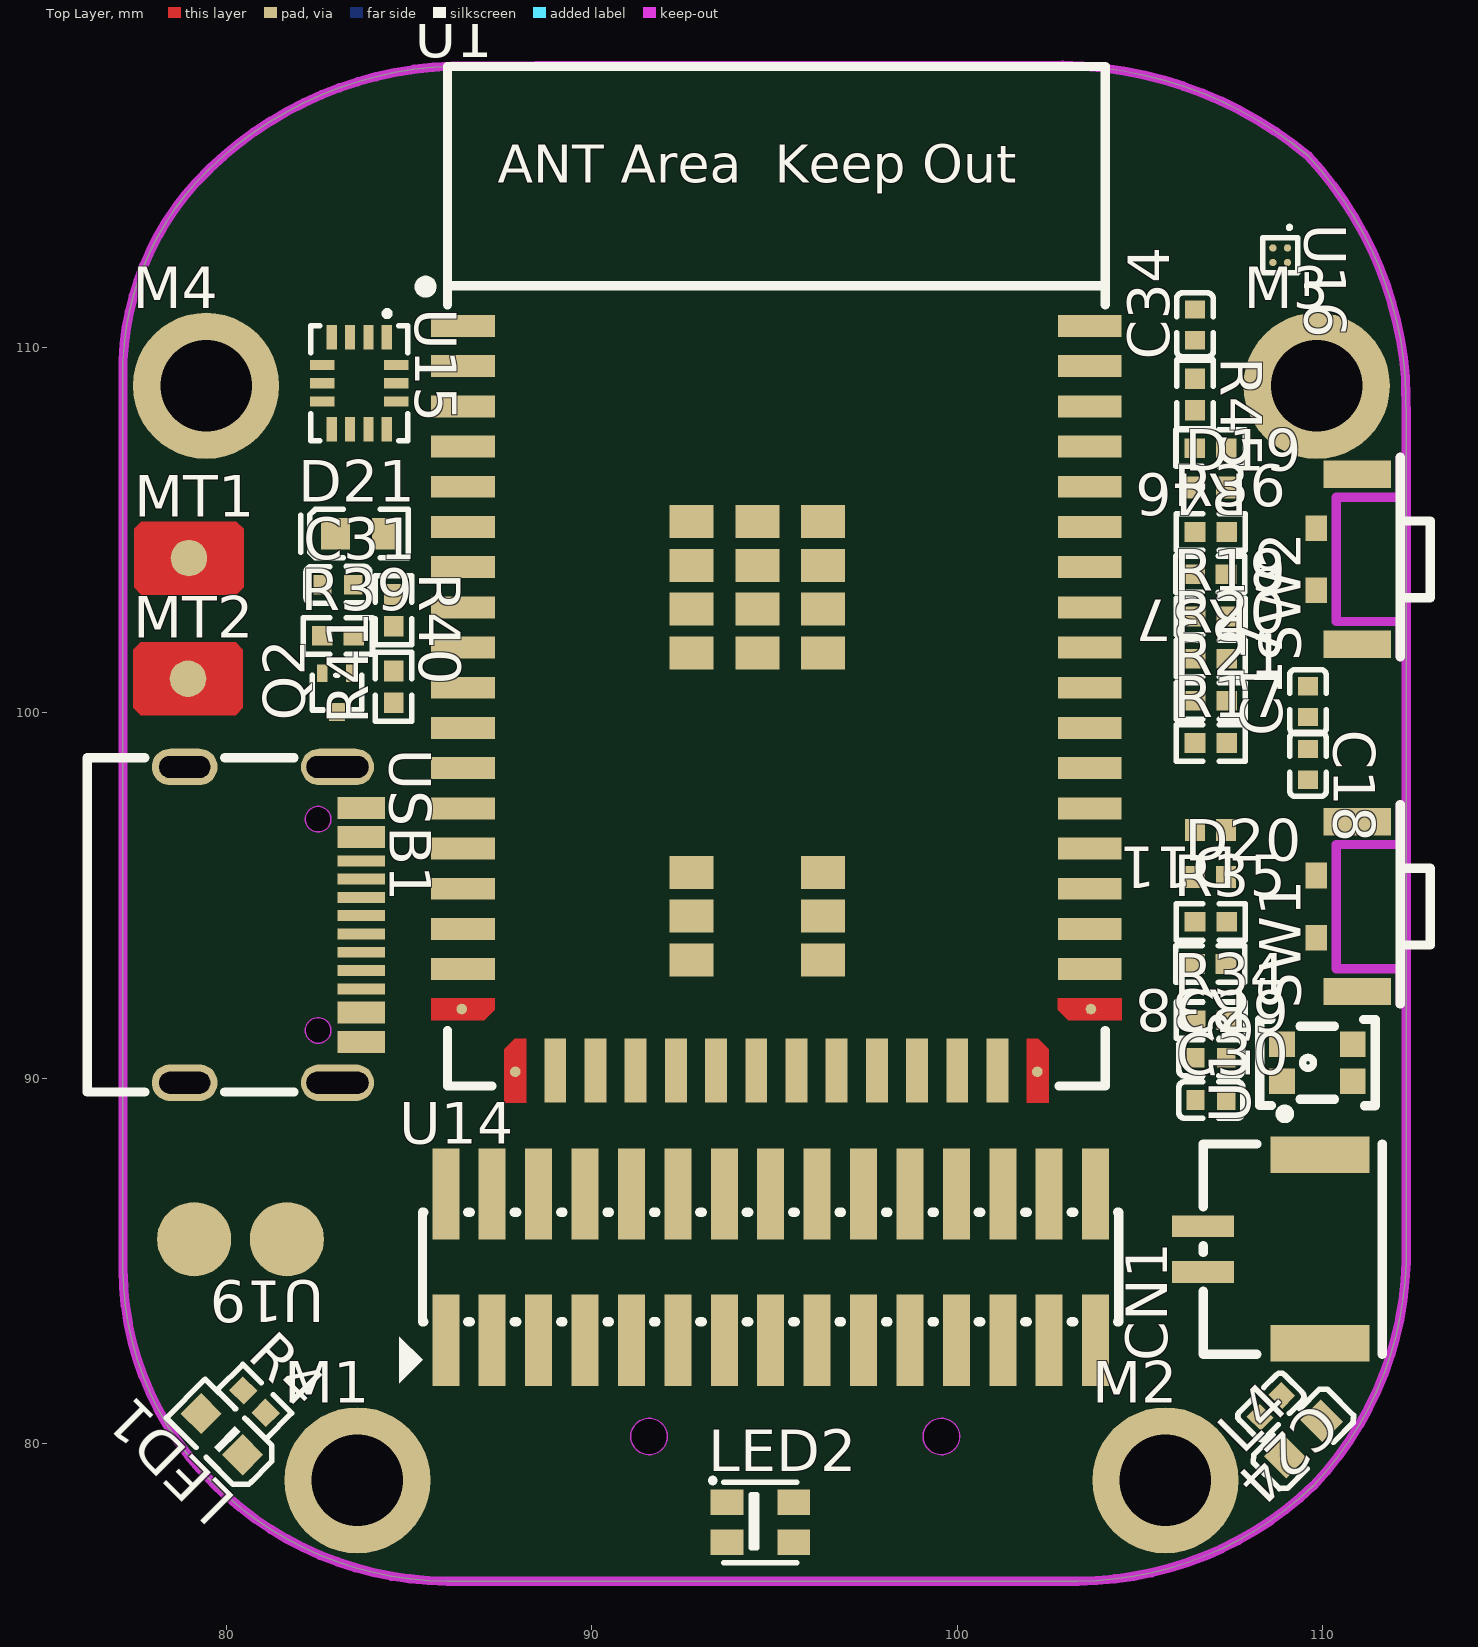
[diagram p0: Top Layer view]
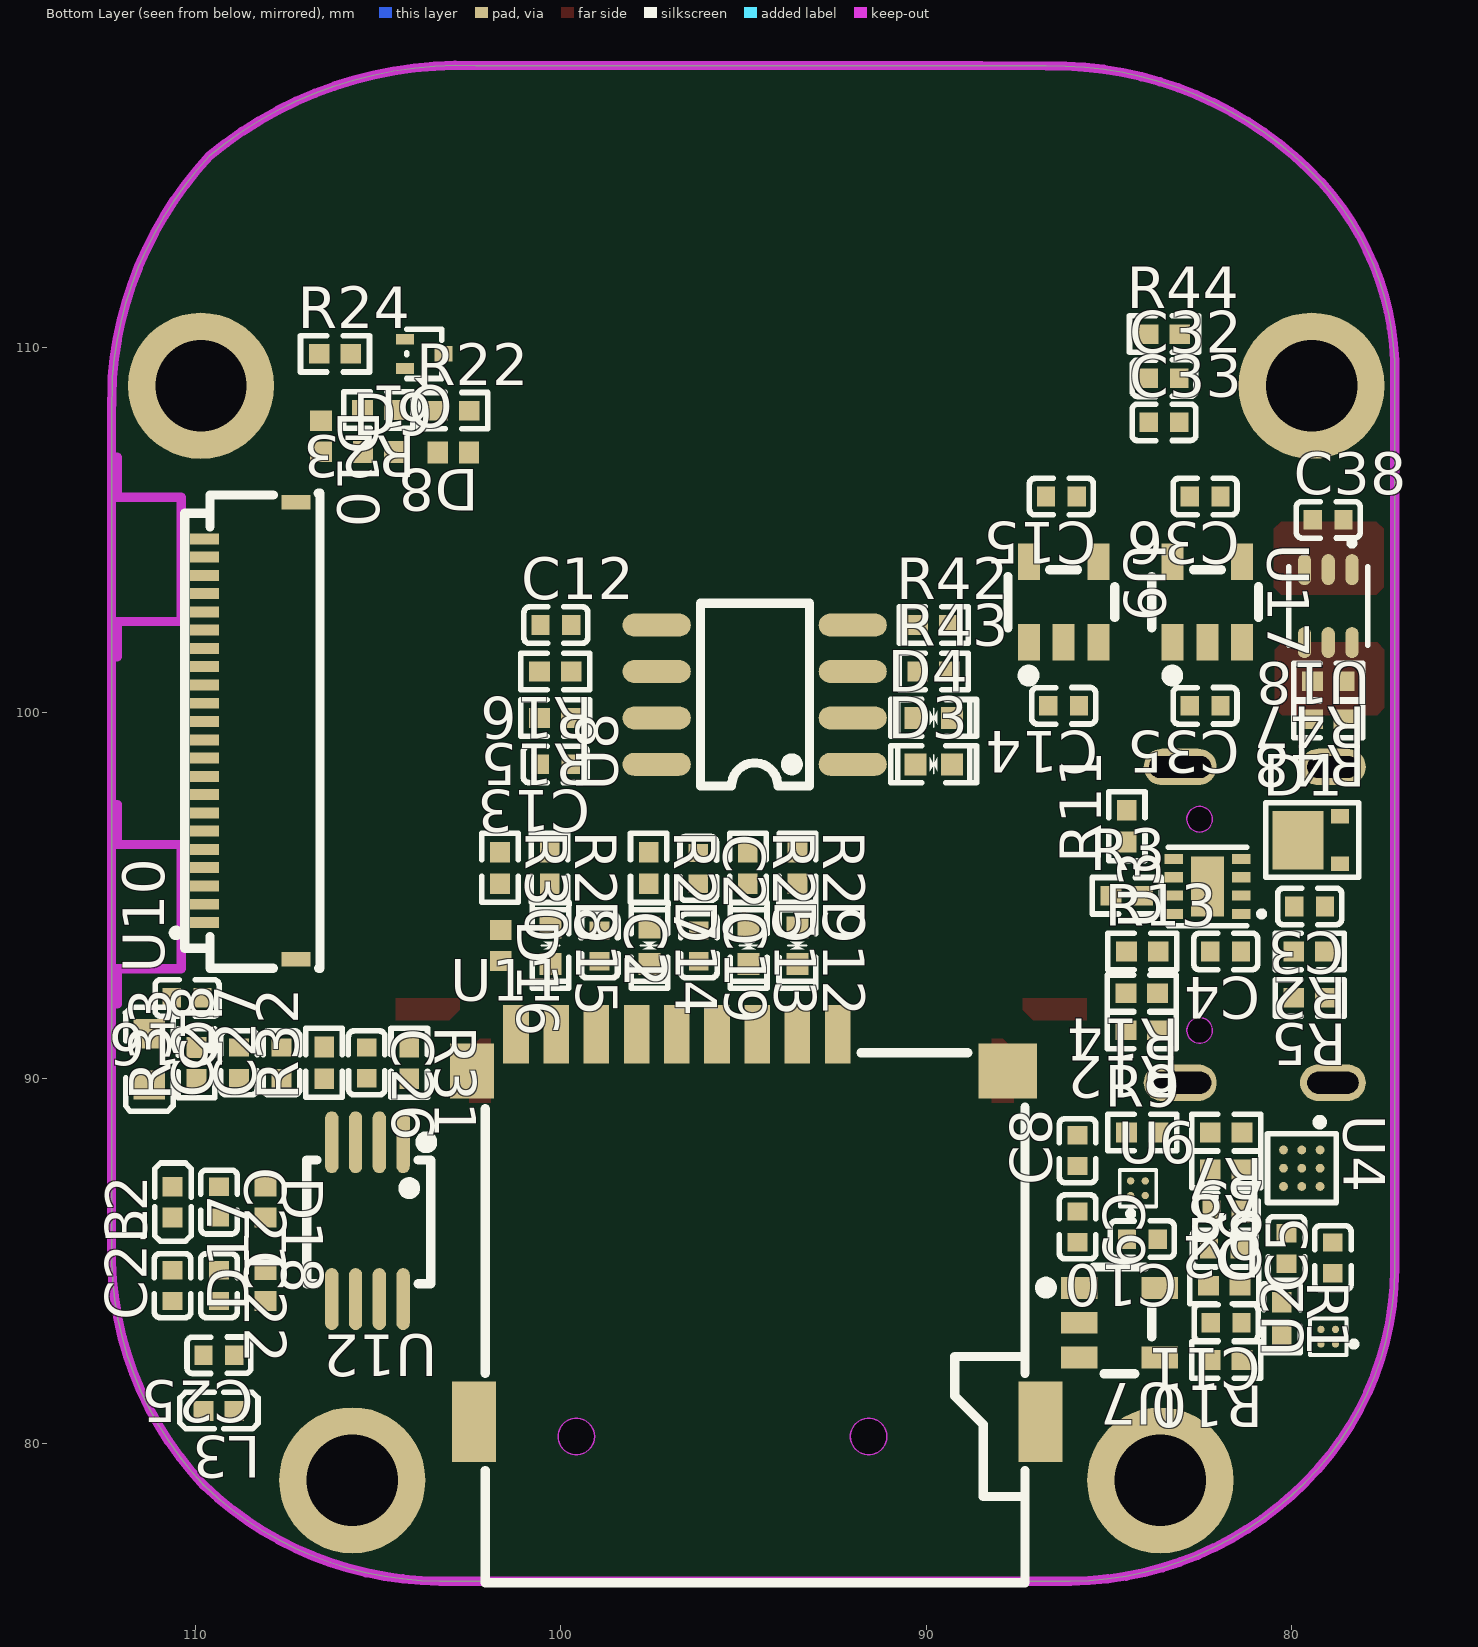
[diagram p1: Bottom Layer view, seen from below]
# Altium PCB MISC52032.pcbdoc
Units mm, origin at the board's own origin, x right, y up, seen from the top; angles counter-clockwise.
Board outline 35.11 x 41.48 mm, 2 copper layers (Top Layer, Bottom Layer), stack 1.58 mm thick; 138 components, 108 nets, 485 pads, 0 vias.

## Layer stack, top to bottom
Top Solder Mask Layer: solder mask 0.01, Dk 3.3
Top Layer: signal copper 0.035
Dielectric1: surface 1.51, FR4, Dk 4.5
Bottom Layer: signal copper 0.035
Bottom Solder Mask Layer: solder mask 0.01, Dk 3.3

## Board outline
103.306,76.242 ccw(c103.243,85.654) 109.749,78.852 ccw(c103.034,85.222) 112.286,84.972 112.286,108.12 112.266,109.185 ccw(c102.232,108.39) 109.606,115.241 ccw(c102.733,106.949) 102.324,117.712 88.477,117.712 86.706,117.702 ccw(c86.519,107.658) 79.185,114.524 ccw(c84.934,109.304) 77.176,109.638 77.176,85.176 ccw(c77.18,85.174) 77.176,85.172 77.176,84.781 ccw(c85.448,84.817) 79.624,78.943 ccw(c86.097,85.346) 86.048,76.242 103.306,76.242

## Design rules (kind name [scope] priority, off if disabled: settings)
BoardOutlineClearance copperThickness2oz_1 [All] p2 off: genericclearance=0.203 ignorepadtopadclearanceinfootprint=FALSE except(0: Arc-SplitContinuation Track-SplitContinuation SMDPad-SplitContinuation THPad-SplitContinuation Via-SplitContinuation Fill-SplitContinuation Region-SplitContinuation Poly-SplitContinuation Text-SplitContinuation Hole-SplitContinuation; 0.152: Arc-CutoutEdge Track-CutoutEdge SMDPad-CutoutEdge THPad-CutoutEdge Via-CutoutEdge Text-CutoutEdge; 0.175: Hole-OutlineEdge Hole-CutoutEdge; 0.254: Poly-OutlineEdge Poly-CutoutEdge; 0.3: Arc-OutlineEdge Track-OutlineEdge SMDPad-OutlineEdge THPad-OutlineEdge Via-OutlineEdge Fill-OutlineEdge Region-OutlineEdge Text-OutlineEdge Fill-CutoutEdge Region-CutoutEdge)
BoardOutlineClearance Plane_innerPlane_1 [All] p4 off: genericclearance=0.102 ignorepadtopadclearanceinfootprint=FALSE except(0: Arc-SplitContinuation Track-SplitContinuation SMDPad-SplitContinuation THPad-SplitContinuation Via-SplitContinuation Fill-SplitContinuation Region-SplitContinuation Poly-SplitContinuation Text-SplitContinuation Hole-SplitContinuation; 0.152: Arc-CutoutEdge Track-CutoutEdge SMDPad-CutoutEdge THPad-CutoutEdge Via-CutoutEdge Text-CutoutEdge; 0.175: Hole-OutlineEdge Hole-CutoutEdge; 0.254: Poly-OutlineEdge Poly-CutoutEdge; 0.3: Arc-OutlineEdge Track-OutlineEdge SMDPad-OutlineEdge THPad-OutlineEdge Via-OutlineEdge Fill-OutlineEdge Region-OutlineEdge Text-OutlineEdge Fill-CutoutEdge Region-CutoutEdge)
BoardOutlineClearance Copper_copperRegion_1 [All] p6 off: genericclearance=0.102 ignorepadtopadclearanceinfootprint=FALSE except(0: Arc-SplitContinuation Track-SplitContinuation SMDPad-SplitContinuation THPad-SplitContinuation Via-SplitContinuation Fill-SplitContinuation Region-SplitContinuation Poly-SplitContinuation Text-SplitContinuation Hole-SplitContinuation; 0.152: Arc-CutoutEdge Track-CutoutEdge SMDPad-CutoutEdge THPad-CutoutEdge Via-CutoutEdge Text-CutoutEdge; 0.175: Hole-OutlineEdge Hole-CutoutEdge; 0.254: Poly-OutlineEdge Poly-CutoutEdge; 0.3: Arc-OutlineEdge Track-OutlineEdge SMDPad-OutlineEdge THPad-OutlineEdge Via-OutlineEdge Fill-OutlineEdge Region-OutlineEdge Text-OutlineEdge Fill-CutoutEdge Region-CutoutEdge)
BoardOutlineClearance copperThickness1oz_1 [All] p8: genericclearance=0.102 ignorepadtopadclearanceinfootprint=FALSE except(0: Arc-SplitContinuation Track-SplitContinuation SMDPad-SplitContinuation THPad-SplitContinuation Via-SplitContinuation Fill-SplitContinuation Region-SplitContinuation Poly-SplitContinuation Text-SplitContinuation Hole-SplitContinuation; 0.152: Arc-CutoutEdge Track-CutoutEdge SMDPad-CutoutEdge THPad-CutoutEdge Via-CutoutEdge Text-CutoutEdge; 0.175: Hole-OutlineEdge Hole-CutoutEdge; 0.254: Poly-OutlineEdge Poly-CutoutEdge; 0.3: Arc-OutlineEdge Track-OutlineEdge SMDPad-OutlineEdge THPad-OutlineEdge Via-OutlineEdge Fill-OutlineEdge Region-OutlineEdge Text-OutlineEdge Fill-CutoutEdge Region-CutoutEdge)
Clearance copperThickness2oz [All] p1 off: gap=0.203 ignorepadtopadclearanceinfootprint=FALSE except(0.152: SMDPad-Track SMDPad-SMDPad THPad-Track SMDPad-THPad THPad-THPad Track-Via SMDPad-Via THPad-Via Via-Via Fill-SMDPad Region-SMDPad Fill-THPad Region-THPad Fill-Via Region-Via Fill-Fill Fill-Region Region-Region Arc-Track Arc-SMDPad Arc-THPad Arc-Via Fill-Arc Region-Arc Arc-Arc Text-Track SMDPad-Text Text-THPad Text-Via Fill-Text Region-Text Arc-Text Text-Text; 0.175: Hole-Track Hole-SMDPad Hole-THPad Hole-Via Fill-Hole Region-Hole Hole-Arc Hole-Text; 0.254: Poly-Track Poly-SMDPad Poly-THPad Poly-Via Poly-Fill Poly-Region Poly-Poly Poly-Arc Poly-Text Poly-Hole; 0.3: Fill-Track Region-Track)
Clearance Plane_innerPlane [All] p3 off: gap=0.102 ignorepadtopadclearanceinfootprint=FALSE except(0.152: SMDPad-Track SMDPad-SMDPad THPad-Track SMDPad-THPad THPad-THPad Track-Via SMDPad-Via THPad-Via Via-Via Fill-SMDPad Region-SMDPad Fill-THPad Region-THPad Fill-Via Region-Via Fill-Fill Fill-Region Region-Region Arc-Track Arc-SMDPad Arc-THPad Arc-Via Fill-Arc Region-Arc Arc-Arc Text-Track SMDPad-Text Text-THPad Text-Via Fill-Text Region-Text Arc-Text Text-Text; 0.175: Hole-Track Hole-SMDPad Hole-THPad Hole-Via Fill-Hole Region-Hole Hole-Arc Hole-Text; 0.254: Poly-Track Poly-SMDPad Poly-THPad Poly-Via Poly-Fill Poly-Region Poly-Poly Poly-Arc Poly-Text Poly-Hole; 0.3: Fill-Track Region-Track)
Clearance Copper_copperRegion [All] p5 off: gap=0.102 ignorepadtopadclearanceinfootprint=FALSE except(0.152: SMDPad-Track SMDPad-SMDPad THPad-Track SMDPad-THPad THPad-THPad Track-Via SMDPad-Via THPad-Via Via-Via Fill-SMDPad Region-SMDPad Fill-THPad Region-THPad Fill-Via Region-Via Fill-Fill Fill-Region Region-Region Arc-Track Arc-SMDPad Arc-THPad Arc-Via Fill-Arc Region-Arc Arc-Arc Text-Track SMDPad-Text Text-THPad Text-Via Fill-Text Region-Text Arc-Text Text-Text; 0.175: Hole-Track Hole-SMDPad Hole-THPad Hole-Via Fill-Hole Region-Hole Hole-Arc Hole-Text; 0.254: Poly-Track Poly-SMDPad Poly-THPad Poly-Via Poly-Fill Poly-Region Poly-Poly Poly-Arc Poly-Text Poly-Hole; 0.3: Fill-Track Region-Track)
Clearance copperThickness1oz [All] p7: gap=0.102 ignorepadtopadclearanceinfootprint=FALSE except(0.152: SMDPad-Track SMDPad-SMDPad THPad-Track SMDPad-THPad THPad-THPad Track-Via SMDPad-Via THPad-Via Via-Via Fill-SMDPad Region-SMDPad Fill-THPad Region-THPad Fill-Via Region-Via Fill-Fill Fill-Region Region-Region Arc-Track Arc-SMDPad Arc-THPad Arc-Via Fill-Arc Region-Arc Arc-Arc Text-Track SMDPad-Text Text-THPad Text-Via Fill-Text Region-Text Arc-Text Text-Text; 0.175: Hole-Track Hole-SMDPad Hole-THPad Hole-Via Fill-Hole Region-Hole Hole-Arc Hole-Text; 0.254: Poly-Track Poly-SMDPad Poly-THPad Poly-Via Poly-Fill Poly-Region Poly-Poly Poly-Arc Poly-Text Poly-Hole; 0.3: Fill-Track Region-Track)
DiffPairsRouting differentialPair [All] p1: maxlimit=0.152 minlimit=0.152 mostfreqgap=0.152 toplayer_minwidth=0.127 toplayer_prefwidth=0.254 toplayer_maxwidth=2.54 toplayer_mingap=0.152 toplayer_prefgap=0.152 toplayer_maxgap=0.152 bottomlayer_minwidth=0.127 bottomlayer_prefwidth=0.254 bottomlayer_maxwidth=2.54 bottomlayer_mingap=0.152 bottomlayer_prefgap=0.152 bottomlayer_maxgap=0.152 maxuncoupledlength=0.254
HoleToHoleClearance otherClearance [All] p1: gap=0.3 allowstackedmicrovias=TRUE
Length netLength [All] p1: minlimit=0 maxlimit=0
PasteMaskExpansion pasteMaskExpansion [All] p1: expansion=0
PlaneConnect innerPlane [All] p1: planeconnectstyle=Relief reliefexpansion=0.508 reliefentries=4 reliefconductorwidth=0.254 reliefairgap=0.254
PolygonConnect copperRegion [All] p1: connectstyle=Relief reliefconductorwidth=0.254 reliefentries=4 polygonreliefangle="90 Angle" airgapwidth=0.254 via.connectstyle=Relief via.reliefconductorwidth=0.254 via.reliefentries=4 via.polygonreliefangle="90 Angle" via.airgapwidth=0.254
RoutingVias viaSize [All] p1: holewidth=0.305 width=0.61 viastyle="Through Hole" minholewidth=0.3 minwidth=0.5 maxholewidth=6.3 maxwidth=10
SolderMaskExpansion solderMaskExpansion [IsVia] p1: expansion=-25.4 istentingtop=TRUE
SolderMaskExpansion solderMaskExpansion [All] p2: expansion=0.051 istentingtop=FALSE
Width copperThickness2oz_2 [All] p1 off: maxlimit=2.54 minlimit=0.203 preferedwidth=0.254
Width copperThickness1oz_2 [All] p2: maxlimit=2.54 minlimit=0.127 preferedwidth=0.254

## Components (designator, comment, footprint, x,y, rotation, side; value= is the part's Value field where it differs from the comment)
C1 "1uF" C0402 98.943,93.625 r270 bottom
C2 "4.7uF" C0402 98.926,93.625 r270 bottom
C3 "1uF" C0402 79.502,94.704 r0 bottom
C4 "4.7uF" C0402 81.799,93.472 r0 bottom
C5 "10uF" C0402 78.867,85.09 r90 bottom
C6 "4.7uF" C0402 80.137,85.344 r90 bottom
C7 "1uF" C0402 81.839,85.344 r180 bottom
C8 "1uF" C0402 85.852,88.019 r90 bottom
C9 "1uF" C0402 85.852,85.936 r270 bottom
C10 "1uF" C0402 84.082,85.598 r0 bottom
C11 "1uF" C0402 81.788,83.312 r0 bottom
C12 "1uF" C0402 100.128,102.402 r180 bottom
C13 "100nF" C0402 100.144,98.592 r0 bottom
C14 "1uF" C0402 86.233,100.194 r0 bottom
C15 "1uF" C0402 86.297,105.918 r0 bottom
C16 "1uF" C0402 110.218,92.202 r0 bottom
C17 "100nF" C0402 109.601,100.31 r90 top
C18 "4.7uF" C0402 109.601,98.59 r270 top
C19 "1uF" C0402 96.216,93.625 r270 bottom
C20 "100nF" C0402 96.231,95.743 r270 bottom
C21 "330pF" C0402 109.347,86.614 r270 bottom
C22 "330pF" C0402 109.347,84.328 r270 bottom
C23 "330pF" C0402 110.617,84.328 r90 bottom
C24 "100nF" C0402 108.585,81.026 r225 top
C25 "22uF" C0402 109.347,82.423 r0 bottom
C26 "1uF" C0402 105.304,90.424 r270 bottom
C27 "100nF" C0402 107.633,90.424 r90 bottom
C28 "100nF" C0402 108.798,90.424 r90 bottom
C29 "4.7uF" C0402 106.942,90.563 r0 top
C30 "10nF" C0402 106.942,89.408 r0 top
C31 "4.7uF" C0402 83.058,103.505 r0 top
C32 "100nF" C0402 83.488,109.157 r180 bottom
C33 "100nF" C0402 83.488,107.95 r180 bottom
C34 "100nF" C0402 106.509,110.617 r90 top
C35 "1uF" C0402 82.364,100.194 r0 bottom
C36 "1uF" C0402 82.364,105.918 r0 bottom
C38 "100nF" C0402 78.994,105.283 r180 bottom
CN1 "A1257WR-S-2P" CONN-SMD_A1257WR-S-2P 108.331,85.328 r90 top locked
D1 "PTVSHC3N18VU" DFN-3_L2.0-W2.0-P1.30-BR 79.248,96.52 r180 bottom locked
D2 "PESDHC2FD12VU" DFN1006-2L-RD 81.788,86.36 r0 bottom
D3 "" D0402-BI 89.789,98.592 r180 bottom
D4 "" D0402-BI 89.789,99.862 r180 bottom
D8 "ESD5451N" DFN1006-2L-BI 102.934,107.125 r0 bottom
D9 "ESD5451N" DFN1006-2L-BI 104.984,107.143 r180 bottom
D10 "ESD5451N" DFN1006-2L-BI 106.553,107.569 r270 bottom
D11 "ESD5451N" DFN1006-2L-BI 106.934,96.796 r180 top
D12 "" D0402-BI 93.519,93.633 r270 bottom
D13 "" D0402-BI 94.855,93.633 r270 bottom
D14 "" D0402-BI 97.565,93.633 r270 bottom
D15 "" D0402-BI 100.275,93.633 r270 bottom
D16 "ESD5451N" DFN1006-2L-BI 101.636,93.633 r270 bottom
D17 "ESD5451N" DFN1006-2L-BI 108.077,84.328 r90 bottom
D18 "ESD5451N" DFN1006-2L-BI 108.077,86.614 r270 bottom
D19 "ESD5451N" DFN1006-2L-BI 106.934,106.172 r0 top
D20 "ESD5451N" DFN1006-2L-BI 106.934,95.505 r0 top
D21 "CD4148WTP" D0603-RD 83.693,104.902 r0 top
L2 "" L0402 110.617,86.614 r90 bottom
L3 "" L0402 109.347,80.899 r0 bottom
L4 "" L0603 109.474,80.137 r45 top
L5 "" L0603 111.252,90.52 r270 bottom
LED1 "" LED0603-RD_GREEN 79.883,80.264 r135 top locked
LED2 "WS2812B-2020" LED-SMD_4P-L2.0-W2.0-TL_WS2812B-2020 94.613,77.851 r0 top locked
M1 "M2-TH" M2_TH_4_2.5MM 83.589,79 r0 top locked
M2 "M2-TH" M2_TH_4_2.5MM 105.699,79 r0 top locked
M3 "M2-TH" M2_TH_4_2.5MM 109.839,108.95 r0 top locked
M4 "M2-TH" M2_TH_4_2.5MM 79.449,108.95 r0 top locked
MT1 "" TP-3x2MM 78.98,104.236 r0 top locked
MT2 "" TP-3x2MM 78.955,100.934 r0 top locked
Q1 "CJ3134K KF" SOT-723_L1.2-W0.8-P0.40-LS1.2-BR 103.729,109.825 r0 bottom locked
Q2 "CJ3134K KF" SOT-723_L1.2-W0.8-P0.40-LS1.2-BR 83.028,100.554 r90 top locked
R1 "100kΩ" R0402 80.264,83.439 r270 bottom
R2 "510kΩ" R0402 79.502,93.472 r0 bottom
R3 "20kΩ" R0402 84.506,94.996 r180 bottom
R4 "4.7kΩ" R0402 80.772,81.153 r315 top
R5 "100kΩ" R0402 79.502,92.202 r0 bottom
R6 "100kΩ" R0402 81.839,84.328 r180 bottom
R7 "2.2kΩ" R0402 81.788,88.519 r0 bottom
R8 "2.2kΩ" R0402 81.788,87.503 r0 bottom
R9 "5.1MΩ" R0402 84.082,88.519 r180 bottom
R10 "5.1MΩ" R0402 81.788,82.296 r0 bottom
R11 "5.1kΩ" R0402 84.506,96.901 r90 bottom
R12 "5.1kΩ" R0402 84.097,91.313 r0 bottom
R13 "390kΩ" R0402 84.082,93.472 r180 bottom
R14 "510kΩ" R0402 84.097,92.329 r0 bottom
R15 "100Ω" R0402 100.144,99.862 r0 bottom
R16 "100Ω" R0402 100.144,101.132 r0 bottom
R17 "22Ω" R0402 106.942,99.174 r0 top
R18 "22Ω" R0402 106.942,102.639 r0 top
R19 "22Ω" R0402 106.942,102.639 r0 top
R20 "22Ω" R0402 106.942,101.484 r0 top
R21 "22Ω" R0402 106.942,100.329 r0 top
R22 "2.2kΩ" R0402 102.934,108.268 r180 bottom
R23 "2.2kΩ" R0402 104.984,108.286 r0 bottom
R24 "2.2kΩ" R0402 106.172,109.825 r180 bottom
R25 "22Ω" R0402 94.875,95.758 r270 bottom
R27 "22Ω" R0402 97.587,95.758 r270 bottom
R28 "22Ω" R0402 100.299,95.758 r270 bottom
R29 "22Ω" R0402 93.519,95.758 r270 bottom
R30 "22Ω" R0402 101.655,95.758 r270 bottom
R31 "5.1MΩ" R0402 104.14,90.424 r270 bottom
R32 "43.2kΩ" R0402 106.469,90.424 r90 bottom
R33 "43.2kΩ" R0402 109.962,90.409 r90 bottom
R34 "1kΩ" R0402 106.942,91.591 r0 top
R35 "5.1kΩ" R0402 106.942,94.282 r0 top
R36 "5.1kΩ" R0402 106.942,104.949 r0 top
R37 "15kΩ" R0402 106.926,103.794 r180 top
R38 "15kΩ" R0402 106.926,93.127 r180 top
R39 "5.1Ω" R0402 83.058,102.108 r0 top
R40 "1.5MΩ" R0402 84.582,102.807 r270 top
R41 "1kΩ" R0402 84.582,100.711 r90 top
R42 "22Ω" R0402 89.789,102.402 r180 bottom
R43 "22Ω" R0402 89.789,101.132 r180 bottom
R44 "2.2kΩ" R0402 83.488,110.363 r180 bottom
R45 "2.2kΩ" R0402 106.509,108.712 r270 top
R46 "2.2kΩ" R0402 106.934,107.243 r180 top
R47 "5.1MΩ" R0402 78.994,100.863 r0 bottom
R48 "22Ω" R0402 78.994,99.822 r0 bottom
SW1 "" KEY-SMD_GT-TC191A-H026-L60 110.389,94.7 r90 top
SW2 "" KEY-SMD_GT-TC191A-H026-L60 110.389,104.2 r90 top locked
U1 "" COMM-SMD_L27.9-W18.0-P1.10_SF32LB52-MOD-1-N16R8 95.054,100.4 r0 top locked
U2 "LP5240HVF" WLCSP-4_L0.8-W0.8-R2-C2-P0.40-BL 78.994,82.931 r90 bottom locked
U3 "LP5305AQVF" DFN-8_L2.0-W2.0-P0.50-BL-EP 82.296,95.25 r90 bottom locked
U4 "AW32001ECSR" WLCSP-9_L1.7-W1.7-R3-C3-P0.50-TL 79.718,87.541 r270 bottom locked
U6 "LP5240HVF" WLCSP-4_L0.8-W0.8-R2-C2-P0.40-BL 84.201,86.994 r180 bottom
U7 "ETA5055V330DS2F" SOT-23-5_L2.9-W1.6-P0.95-LS2.8-BR 84.709,83.312 r0 bottom locked
U8 "CH340N" SOP-8_L4.9-W3.9-P1.27-LS6.0-BL 94.687,100.497 r90 bottom locked
U9 "ETA5055V330DS2F" SOT-23-5_L2.9-W1.6-P0.95-LS2.8-BR 86.233,103.031 r270 bottom locked
U10 "AFH34-S22FIA-1H" FPC-SMD_22P-P0.50_JS_AFH34-S22FIA-1H 108.489,99.513 r90 bottom locked
U11 "TF-115Y-ACP9" SIM-SMD_TF-115Y-BCP9 94.644,85.9 r180 bottom locked
U12 "NS4150B" MSOP-8_L3.0-W3.0-P0.65-LS5.0-BL 105.283,86.106 r0 bottom locked
U13 "LMA2718T421-OA5" MIC-SMD_4P-L2.8-W1.9-P1.01-TL 109.855,90.424 r90 top locked
U14 "XDZ127-2-15-S-1.0-G1" HDR-SMD_30P-P1.27-V-M-R2-C15-LS5.5_1 94.899,84.836 r0 top locked
U15 "LSM6DS3TR-C" LGA-14_L3.0-W2.5-P0.50-TL 83.64,109.019 r270 top locked
U16 "MMC5603NJ" FLIPCHIP-4_L0.8-W0.8-R2-C2-P0.40-TL 108.839,112.522 r270 top
U17 "ETA5055V330DS2F" SOT-23-5_L2.9-W1.6-P0.95-LS2.8-BR 82.301,103.031 r270 bottom locked
U18 "LTR-303ALS-01" TDFN-6_L2.0-W2.0-P0.65-BL 78.994,102.921 r0 bottom locked
U19 "" 焊盘 81.661,85.598 r180 top locked
USB1 "KH-TYPE-C-16P" USB-C-SMD_KH-TYPE-C-16P 81.28,94.2 r270 top locked

## Footprints (in the part's own frame and the unit in brackets; to place one, negate y for a bottom-side part, rotate by r counter-clockwise, add the part's x,y. Pads: shape width x height; smd on the part's side, far side on the other; paste and mask are expansions set on the pad)
C0402 [mm]
  rect 0.5x0.54 smd: 1(-0.42,0) 2(0.42,0)
  silkscreen extent -0.87,-0.5 0.87,0.5
COMM-SMD_L27.9-W18.0-P1.10_SF32LB52-MOD-1-N16R8 [mm]
  rect 1.75x0.6 smd paste+0 mask+0.05: 1(-8.575,10.188) 2(-8.575,9.087) 3(-8.575,7.988) 4(-8.575,6.888) 5(-8.575,5.788) 6(-8.575,4.687) 7(-8.575,3.588) 8(-8.575,2.488) 9(-8.575,1.387) 10(-8.575,0.288) 11(-8.575,-0.812) 12(-8.575,-1.912) 13(-8.575,-3.012) 14(-8.575,-4.112) 15(-8.575,-5.212) 16(-8.575,-6.313) 17(-8.575,-7.412) 32(8.575,-7.412) 33(8.575,-6.313) 34(8.575,-5.212) 35(8.575,-4.112) 36(8.575,-3.012) 37(8.575,-1.912) 38(8.575,-0.812) 39(8.575,0.288) 40(8.575,1.387) 41(8.575,2.488) 42(8.575,3.588) 43(8.575,4.687) 44(8.575,5.788) 45(8.575,6.888) 46(8.575,7.988) 47(8.575,9.087) 48(8.575,10.188)
  round 0.292 smd: 18(-8.607,-8.504) 31(8.607,-8.504) 61(-7.142,-10.22) 62(7.142,-10.22)
  rect 0.6x1.75 smd paste+0 mask+0.05: 19(-6.05,-10.188) 20(-4.95,-10.188) 21(-3.85,-10.188) 22(-2.75,-10.188) 23(-1.65,-10.188) 24(-0.55,-10.188) 25(0.55,-10.188) 26(1.65,-10.188) 27(2.75,-10.188) 28(3.85,-10.188) 29(4.95,-10.188) 30(6.05,-10.188)
  rect 1.2x0.9 smd paste+0 mask+0.05: 49(-2.32,4.838) 50(-0.52,4.838) 51(1.28,4.838) 52(-2.32,3.638) 53(-0.52,3.638) 54(1.28,3.638) 55(-2.32,2.438) 56(-0.52,2.438) 57(1.28,2.438) 58(-2.32,1.238) 59(-0.52,1.238) 60(1.28,1.238) 63(-2.32,-4.762) 64(-2.32,-5.963) 65(-2.32,-7.162) 66(1.28,-4.762) 67(1.28,-5.963) 68(1.28,-7.162)
  Top Layer region: 7.7,-8.213 7.7,-8.523 7.99,-8.813 8.025,-8.813 8.025,-8.813 9.125,-8.813 9.125,-8.813 9.45,-8.813 9.45,-8.213
  Top Layer region: 6.85,-9.313 6.85,-11.063 7.45,-11.063 7.45,-10.738 7.45,-10.738 7.45,-9.638 7.45,-9.638 7.45,-9.603 7.16,-9.313
  Top Layer region: -6.85,-11.063 -6.85,-9.313 -7.16,-9.313 -7.45,-9.603 -7.45,-9.638 -7.45,-9.638 -7.45,-10.738 -7.45,-10.738 -7.45,-11.063
  Top Layer region: -7.7,-8.522 -7.7,-8.213 -9.45,-8.213 -9.45,-8.813 -9.125,-8.813 -8.025,-8.813 -7.99,-8.813
  silkscreen extent -9.75,-10.61 9,17.29
CONN-SMD_A1257WR-S-2P [mm]
  rect 0.6x1.7 smd: 1(0.625,1.6) 2(-0.625,1.6)
  rect 1x2.7 smd: 3(2.575,-1.6) 4(-2.575,-1.6)
  silkscreen extent -2.88,-3.3 2.87,1.6
D0402-BI [mm]
  rect 0.6x0.6 smd paste-100 mask+0.051: 1(-0.5,0) 2(0.5,0)
  silkscreen extent -1.18,-0.5 1.17,0.51
D0603-RD [mm]
  rect 0.8x0.864 smd paste-100 mask+0.051: 1(-0.7,0) 2(0.7,0)
  silkscreen extent -1.65,-0.65 1.28,0.67
DFN1006-2L-BI [mm]
  rect 0.55x0.6 smd paste+0 mask+0.051: 1(-0.425,0) 2(0.425,0)
DFN1006-2L-RD [mm]
  rect 0.5x0.6 smd: 1(-0.4,0) 2(0.4,0)
  silkscreen extent -0.9,-0.5 0.8,0.5
DFN-3_L2.0-W2.0-P1.30-BR [mm]
  rect 0.5x0.4 smd: 1(0.575,-0.65) 2(0.575,0.65)
  rect 1.4x1.6 smd: 3(-0.575,0)
  silkscreen extent -1.46,-1.02 1.08,1.02
DFN-8_L2.0-W2.0-P0.50-BL-EP [mm]
  rect 0.28x0.505 smd: 1(-0.75,-0.928) 2(-0.25,-0.928) 3(0.25,-0.928) 4(0.75,-0.928) 5(0.75,0.928) 6(0.25,0.928) 7(-0.25,0.928) 8(-0.75,0.928)
  rect 1.65x0.9 smd: 9(0,0)
  silkscreen extent -1.08,-1.55 1.08,1.08
FLIPCHIP-4_L0.8-W0.8-R2-C2-P0.40-TL [mm]
  round 0.2 smd paste-100 mask+0.051: A1(-0.2,0.2) A2(0.2,0.2) B1(-0.2,-0.2) B2(0.2,-0.2)
  silkscreen extent -0.81,-0.48 0.48,0.48
FPC-SMD_22P-P0.50_JS_AFH34-S22FIA-1H [mm]
  rect 0.3x0.8 smd paste+0 mask+0.05: 1(-5.25,1.25) 2(-4.75,1.25) 3(-4.25,1.25) 4(-3.75,1.25) 5(-3.25,1.25) 6(-2.75,1.25) 7(-2.25,1.25) 8(-1.75,1.25) 9(-1.25,1.25) 10(-0.75,1.25) 11(-0.25,1.25) 12(0.25,1.25) 13(0.75,1.25) 14(1.25,1.25) 15(1.75,1.25) 16(2.25,1.25) 17(2.75,1.25) 18(3.25,1.25) 19(3.75,1.25) 20(4.25,1.25) 21(4.75,1.25) 22(5.25,1.25)
  rect 0.4x0.8 smd paste+0 mask+0.05: 23(6.25,-1.25) 24(-6.25,-1.25)
  silkscreen extent -6.5,-1.91 6.5,2.13
HDR-SMD_30P-P1.27-V-M-R2-C15-LS5.5_1 [mm]
  rect 0.74x2.5 smd paste+0 mask+0.05: 1(-8.89,-2) 2(-8.89,2) 3(-7.62,-2) 4(-7.62,2) 5(-6.35,-2) 6(-6.35,2) 7(-5.08,-2) 8(-5.08,2) 9(-3.81,-2) 10(-3.81,2) 11(-2.54,-2) 12(-2.54,2) 13(-1.27,-2) 14(-1.27,2) 15(0,-2) 16(0,2) 17(1.27,-2) 18(1.27,2) 19(2.54,-2) 20(2.54,2) 21(3.81,-2) 22(3.81,2) 23(5.08,-2) 24(5.08,2) 25(6.35,-2) 26(6.35,2) 27(7.62,-2) 28(7.62,2) 29(8.89,-2) 30(8.89,2)
  silkscreen extent -10.16,-3.17 9.52,1.5
KEY-SMD_GT-TC191A-H026-L60 [mm]
  rect 0.7x0.6 smd paste+0 mask+0.05: 1(-0.85,0.563) 2(0.85,0.563)
  rect 0.75x1.85 smd paste+0 mask+0.05: 3(-2.325,-0.562) 4(2.325,-0.562)
  Board Outline Layer lines w0.254: -2.667,-1.738 -1.7,-1.738 -1.7,0.012 1.7,0.012 1.7,-1.738 2.794,-1.738
  silkscreen extent -2.67,-2.56 2.79,-1.74
L0402 [mm]
  rect 0.54x0.54 smd: 1(-0.42,0) 2(0.42,0)
  silkscreen extent -1.07,-0.51 1.07,0.49
L0603 [mm]
  rect 0.8x0.864 smd paste-100 mask+0.051: 1(-0.7,0) 2(0.7,0)
  silkscreen extent -1.42,-0.65 1.42,0.65
LED0603-RD_GREEN [mm]
  rect 0.8x0.8 smd: 1(-0.799,-0.003) 2(0.799,0.003)
  silkscreen extent -1.49,-0.75 1.39,0.76
LED-SMD_4P-L2.0-W2.0-TL_WS2812B-2020 [mm]
  rect 0.9x0.7 smd: 1(-0.915,0.55) 2(-0.915,-0.55) 3(0.915,-0.55) 4(0.915,0.55)
  silkscreen extent -1.3,-1.1 1,1.15
LGA-14_L3.0-W2.5-P0.50-TL [mm]
  rect 0.675x0.28 smd: 1(-1.262,0.75) 2(-1.262,0.25) 3(-1.262,-0.25) 4(-1.262,-0.75) 8(1.262,-0.75) 9(1.262,-0.25) 10(1.262,0.25) 11(1.262,0.75)
  rect 0.28x0.675 smd: 5(-0.5,-1.012) 6(0,-1.012) 7(0.5,-1.012) 12(0.5,1.012) 13(0,1.012) 14(-0.5,1.012)
  silkscreen extent -1.98,-1.33 1.58,1.33
M2_TH_4_2.5MM [mm]
  round 4 hole 2.5: 1(0,0)
MIC-SMD_4P-L2.8-W1.9-P1.01-TL [mm]
  rect 0.7x0.7 smd: 1(-0.505,0.965) 2(-0.505,-0.965) 3(0.505,-0.965) 4(0.505,0.965)
  silkscreen extent -1.52,-1.59 1.19,1.58
MSOP-8_L3.0-W3.0-P0.65-LS5.0-BL [mm]
  oval 0.364x1.692 smd: 1(-0.975,-2.146) 2(-0.325,-2.146) 3(0.325,-2.146) 4(0.975,-2.146) 5(0.975,2.146) 6(0.325,2.146) 7(-0.325,2.146) 8(-0.975,2.146)
  silkscreen extent -1.76,-2.3 1.66,1.73
R0402 [mm]
  rect 0.566x0.54 smd paste-100 mask+0.051: 1(-0.433,0) 2(0.433,0)
  silkscreen extent -0.94,-0.5 0.94,0.5
SIM-SMD_TF-115Y-BCP9 [mm]
  rect 0.7x1.6 smd: 1(2.225,5.3) 2(1.125,5.3) 3(0.025,5.3) 4(-1.075,5.3) 5(-2.175,5.3) 6(-3.275,5.3) 7(-4.375,5.3) 8(-5.475,5.3) Cd(-6.575,5.3)
  rect 1.2x1.5 smd: 10(-7.775,4.3)
  rect 1.6x1.5 smd: 11(6.875,4.3)
  rect 1.2x2.2 smd: 12(-7.725,-5.3) 13(7.775,-5.3)
  Board Outline Layer circle w0.003: c-4.925,-5.7 r0.5
  Board Outline Layer circle w0.003: c3.075,-5.7 r0.5
  Board Outline Layer region: -5.425,-5.7 -5.375,-5.917 -5.237,-6.091 -5.036,-6.187 -4.814,-6.187 -4.613,-6.091 -4.474,-5.917 -4.425,-5.7 -4.425,-5.7 -4.474,-5.483 -4.613,-5.309 -4.814,-5.213 -5.036,-5.213 -5.237,-5.309 -5.375,-5.483 -5.425,-5.7
  Board Outline Layer region: -5.425,-5.7 -5.415,-5.798 -5.387,-5.891 -5.341,-5.978 -5.278,-6.054 -5.203,-6.116 -5.116,-6.162 -5.022,-6.19 -4.925,-6.2 -4.827,-6.19 -4.734,-6.162 -4.647,-6.116 -4.571,-6.054 -4.509,-5.978 -4.463,-5.891 -4.435,-5.798 -4.425,-5.7 -4.435,-5.602 -4.463,-5.509 -4.509,-5.422 -4.571,-5.346 -4.647,-5.284 -4.734,-5.238 -4.827,-5.21 -4.925,-5.2 -5.022,-5.21 -5.116,-5.238 -5.203,-5.284 -5.278,-5.346 -5.341,-5.422 -5.387,-5.509 -5.415,-5.602
  Board Outline Layer region: 2.575,-5.7 2.625,-5.917 2.763,-6.091 2.964,-6.187 3.186,-6.187 3.387,-6.091 3.526,-5.917 3.575,-5.7 3.575,-5.7 3.526,-5.483 3.387,-5.309 3.186,-5.213 2.964,-5.213 2.763,-5.309 2.625,-5.483 2.575,-5.7
  Board Outline Layer region: 2.575,-5.7 2.585,-5.798 2.613,-5.891 2.659,-5.978 2.721,-6.054 2.797,-6.116 2.884,-6.162 2.978,-6.19 3.075,-6.2 3.173,-6.19 3.266,-6.162 3.353,-6.116 3.429,-6.054 3.491,-5.978 3.537,-5.891 3.565,-5.798 3.575,-5.7 3.565,-5.602 3.537,-5.509 3.491,-5.422 3.429,-5.346 3.353,-5.284 3.266,-5.238 3.173,-5.21 3.075,-5.2 2.978,-5.21 2.884,-5.238 2.797,-5.284 2.721,-5.346 2.659,-5.422 2.613,-5.509 2.585,-5.602
  Multi-Layer board cut-out: -5.425,-5.7 -5.375,-5.917 -5.237,-6.091 -5.036,-6.187 -4.814,-6.187 -4.613,-6.091 -4.474,-5.917 -4.425,-5.7 -4.425,-5.7 -4.474,-5.483 -4.613,-5.309 -4.814,-5.213 -5.036,-5.213 -5.237,-5.309 -5.375,-5.483 -5.425,-5.7
  Multi-Layer board cut-out: 2.575,-5.7 2.625,-5.917 2.763,-6.091 2.964,-6.187 3.186,-6.187 3.387,-6.091 3.526,-5.917 3.575,-5.7 3.575,-5.7 3.526,-5.483 3.387,-5.309 3.186,-5.213 2.964,-5.213 2.763,-5.309 2.625,-5.483 2.575,-5.7
  silkscreen extent -7.42,-9.7 7.35,4.8
SOP-8_L4.9-W3.9-P1.27-LS6.0-BL [mm]
  oval 0.63x1.865 smd: 1(-1.905,-2.682) 2(-0.635,-2.682) 3(0.635,-2.682) 4(1.905,-2.682) 5(1.905,2.682) 6(0.635,2.682) 7(-0.635,2.682) 8(-1.905,2.682)
  silkscreen extent -2.5,-1.5 2.5,1.48
SOT-23-5_L2.9-W1.6-P0.95-LS2.8-BR [mm]
  rect 1x0.6 smd paste+0 mask+0.05: 1(1.1,-0.95) 2(1.1,0) 3(1.1,0.95) 4(-1.1,0.95) 5(-1.1,-0.95)
  silkscreen extent -0.89,-1.52 2.16,1.4
SOT-723_L1.2-W0.8-P0.40-LS1.2-BR [mm]
  rect 0.489x0.294 smd: 1(0.53,-0.4) 2(0.53,0.4)
  rect 0.489x0.434 smd: 3(-0.53,0)
  silkscreen extent -0.48,-0.68 0.48,0.68
TDFN-6_L2.0-W2.0-P0.65-BL [mm]
  oval 0.364x0.847 smd: 1(-0.65,-0.998) 2(0,-0.998) 3(0.65,-0.998) 4(0.65,0.998) 5(0,0.998) 6(-0.65,0.998)
  silkscreen extent -1.08,-1.8 1.08,1.08
TP-3x2MM [mm]
  round 1 smd: 1(0,0)
  Top Layer region: -1.5,-0.8 -1.5,0.8 -1.3,1 1.3,1 1.5,0.8 1.5,-0.8 1.3,-1 -1.3,-1
USB-C-SMD_KH-TYPE-C-16P [mm]
  oval 1x2 hole 0.6 slot 1.7 at 90 deg: 1(-4.32,1.765) 2(4.32,1.765)
  oval 1x1.8 hole 0.6 slot 1.4 at 90 deg: 3(-4.32,-2.415) 4(4.32,-2.415)
  rect 0.3x1.3 smd paste-100 mask+0.05: A1(-3.35,2.415) A4(-2.55,2.415) A5(-1.25,2.415) A6(-0.25,2.415) A7(0.25,2.415) A8(1.25,2.415) A9(2.55,2.415) A12(3.35,2.415) B1(3.05,2.415) B4(2.25,2.415) B5(1.75,2.415) B6(0.75,2.415) B7(-0.75,2.415) B8(-1.75,2.415) B9(-2.25,2.415) B12(-3.05,2.415)
  Board Outline Layer circle w0.003: c-2.89,1.235 r0.35
  Board Outline Layer circle w0.003: c2.89,1.235 r0.35
  Board Outline Layer region: -2.89,1.585 -2.738,1.55 -2.616,1.453 -2.549,1.313 -2.549,1.157 -2.616,1.017 -2.738,0.92 -2.89,0.885 -2.89,0.885 -3.042,0.92 -3.164,1.017 -3.231,1.157 -3.231,1.313 -3.164,1.453 -3.042,1.55 -2.89,1.585
  Board Outline Layer region: -2.89,1.585 -2.812,1.576 -2.738,1.55 -2.672,1.509 -2.616,1.453 -2.575,1.387 -2.549,1.313 -2.54,1.235 -2.549,1.157 -2.575,1.083 -2.616,1.017 -2.672,0.961 -2.738,0.92 -2.812,0.894 -2.89,0.885 -2.968,0.894 -3.042,0.92 -3.108,0.961 -3.164,1.017 -3.205,1.083 -3.231,1.157 -3.24,1.235 -3.231,1.313 -3.205,1.387 -3.164,1.453 -3.108,1.509 -3.042,1.55 -2.968,1.576
  Board Outline Layer region: 2.89,1.585 3.042,1.55 3.164,1.453 3.231,1.313 3.231,1.157 3.164,1.017 3.042,0.92 2.89,0.885 2.89,0.885 2.738,0.92 2.616,1.017 2.549,1.157 2.549,1.313 2.616,1.453 2.738,1.55 2.89,1.585
  Board Outline Layer region: 2.89,1.585 2.968,1.576 3.042,1.55 3.108,1.509 3.164,1.453 3.205,1.387 3.231,1.313 3.24,1.235 3.231,1.157 3.205,1.083 3.164,1.017 3.108,0.961 3.042,0.92 2.968,0.894 2.89,0.885 2.812,0.894 2.738,0.92 2.672,0.961 2.616,1.017 2.575,1.083 2.549,1.157 2.54,1.235 2.549,1.313 2.575,1.387 2.616,1.453 2.672,1.509 2.738,1.55 2.812,1.576
  Multi-Layer board cut-out: -2.89,1.585 -2.738,1.55 -2.616,1.453 -2.549,1.313 -2.549,1.157 -2.616,1.017 -2.738,0.92 -2.89,0.885 -2.89,0.885 -3.042,0.92 -3.164,1.017 -3.231,1.157 -3.231,1.313 -3.164,1.453 -3.042,1.55 -2.89,1.585
  Multi-Layer board cut-out: 2.89,1.585 3.042,1.55 3.164,1.453 3.231,1.313 3.231,1.157 3.164,1.017 3.042,0.92 2.89,0.885 2.89,0.885 2.738,0.92 2.616,1.017 2.549,1.157 2.549,1.313 2.616,1.453 2.738,1.55 2.89,1.585
  silkscreen extent -4.57,-5.08 4.57,0.57
WLCSP-4_L0.8-W0.8-R2-C2-P0.40-BL [mm]
  round 0.2 smd paste-100 mask+0.051: A1(-0.2,-0.2) A2(-0.2,0.2) B1(0.2,-0.2) B2(0.2,0.2)
  silkscreen extent -0.5,-0.78 0.5,0.5
WLCSP-9_L1.7-W1.7-R3-C3-P0.50-TL [mm]
  round 0.24 smd paste-100 mask+0.051: A1(-0.5,0.5) A2(0,0.5) A3(0.5,0.5) B1(-0.5,0) B2(0,0) B3(0.5,0) C1(-0.5,-0.5) C2(0,-0.5) C3(0.5,-0.5)
  silkscreen extent -1.36,-0.94 0.94,0.94
焊盘 [mil]
  round 80 smd: 1(0,0) 2(100,0)

## Nets (pads, with @x,y where several pads share a name; then routed paths per layer and width w, separated by ;. In a path a pad name is that pad's centre, name@x,y a point inside that pad or via, vN(x,y) a via of type N, cw(c..) or ccw(c..) an arc to the next point about the centre after c; other vN are vias at no path point)
$C7_1: C7.1 R5.1 R6.1 U4.B3
$C21_2: C21.2 C23.2 CN1.1 D18.2 L3.2
$C22_1: C22.1 C23.1 CN1.2 D17.2 L2.2
$C24_2: C24.2 C25.2 U12.6
$C26_2: C26.2 U12.2
$C27_1: C27.1 R32.1
$C28_1: C28.1 R33.1
$C29_2: C29.2 R34.1 U13.4
$C31_2: C31.2 D21.1 MT1.1 R39.2
$D12_2: D12.2 R29.2 U11.2
$D13_2: D13.2 R25.2 U11.3
$D15_2: D15.2 R28.2 U11.7
$D16_2: D16.2 R30.2 U11.Cd
$D21_2: D21.2 MT2.1 Q2.3
$L2_1: L2.1 U12.5
$L3_1: L3.1 U12.8
$LED1_2: LED1.2 R4.1
$Q2_1: Q2.1 R40.2 R41.1
$R3_2: R3.2 U3.7
$R5_2: R5.2 U4.B1
$R11_2: R11.2 USB1.A5
$R12_1: R12.1 USB1.B5
$R17_2: R17.2 U10.3
$R18_2: R18.2 U10.4
$R19_2: R19.2 U10.13
$R20_2: R20.2 U10.14
$R21_2: R21.2 U10.16
$R27_2: R27.2 U11.5
$R32_2: R32.2 U12.3
$R33_2: R33.2 U12.4
$R42_2: R42.2 U1.12
$R43_1: R43.1 U1.13
$R47_2: R47.2 R48.2 U17.3
$U17_1: U17.1
ADCIN: C30.2 U1.37 U13.1
CH_3V3: C12.2 C13.1 C15.2 U8.5 U8.8 U9.5
CH_RTS#: R1.1 U2.B2 U8.4
CH_USB_DM: D4.2 U8.2 USB1.A7 USB1.B7
CH_USB_DP: D3.2 U8.1 USB1.A6 USB1.B6
CHG_INT: Q1.3 R6.2 U4.B2
DAC1N: C28.2 U1.34
DAC1P: C27.2 U1.33
GND: C1.1 C2.1 C3.1 C4.1 C5.2 C6.2 C7.2 C8.1 C9.1 C10.1 C11.1 C12.1 C13.2 C14.1 C15.1 C16.2 C17.1 C18.1 C19.1 C20.1 C31.1 C32.2 C33.2 C34.2 C35.1 C36.1 C38.1 D1.1 D1.2 D2.2 D3.1 D4.1 D8.1 D9.1 D10.1 D11.1 D12.1 D13.1 D14.1 D15.1 D16.1 D19.1 D20.1 L4.1 L5.1 LED1.1 LED2.2 M1.1 M2.1 M3.1 M4.1 Q1.2 Q2.2 R2.1 R3.1 R9.1 R10.1 R11.1 R12.2 R14.1 R37.1 R38.1 R40.1 R47.1 SW1.3 SW1.4 SW2.3 SW2.4 U1.1 U1.26 U1.35 U1.48 U1.49 U1.50 U1.51 U1.52 U1.53 U1.54 U1.55 U1.56 U1.57 U1.58 U1.59 U1.60 U2.B1 U3.2 U3.5 U3.6 U3.9 U4.C3 U6.B1 U7.2 U8.3 U9.2 U10.22 U10.23 U10.24 U11.6 U11.10 U11.11 U11.12 U11.13 U12.7 U14.3 U14.4 U14.9 U14.10 U15.1 U15.2 U15.3 U15.6 U15.7 U16.A1 U17.2 U18.3 U19.2 USB1.1 USB1.2 USB1.3 USB1.4 USB1.A1 USB1.A12 USB1.B1 USB1.B12
GS_3V3: C32.1 C33.1 C34.1 C36.2 C38.2 R44.2 R45.2 R46.2 U15.5 U15.8 U15.12 U16.B1 U17.5 U18.1
MIC_BIAS: R34.2 U1.36
MIC_GND: C29.1 C30.1 L5.2 U13.2 U13.3
PA26: R10.2 U7.3
PA30: R48.1
PA31: R44.1 U15.4
PA38: U1.10
PA43_KEY2: D20.2 R35.2 SW1.2
PA_00_LCD_QSPI_RSTB: U1.47 U10.12
PA_01_LCD_BL_PWM: U1.46 U10.2
PA_02_LCD_QSPI_TE: U1.45 U10.11
PA_03_LCD_QSPI_CS: U1.44 U10.15
PA_04_LCD_QSPI_CLK: R19.1 U1.43
PA_05_LCD_QSPI_D0: R20.1 U1.42
PA_06_LCD_QSPI_D1: R21.1 U1.41
PA_07_LCD_QSPI_D2: R17.1 U1.40
PA_08_LCD_QSPI_D3: R18.1 U1.39
PA_09_TP_RSTN: D11.2 U1.38 U10.21
PA_10_I2C2_SCL: R8.2 U1.32 U4.C2 U14.30
PA_11_I2C2_SDA: R7.2 U1.31 U4.C1 U14.29
PA_18_UART_RXD: R16.2 U1.30
PA_19_UART_TXD: R15.2 U1.29
PA_20_VIB_PWM: R41.2 U1.28 U14.24
PA_24_SPI1_DO: R25.1 U1.18
PA_24_SPI1_DO_1: U14.20
PA_25_SPI1_DI: R28.1 U1.19
PA_25_SPI1_DI_1: U14.22
PA_26: U1.20
PA_27_SD_DET: R30.1 U1.21
PA_27_SD_DET_1: U14.23
PA_28_SPI1_CLK: R27.1 U1.22
PA_28_SPI1_CLK_1: U14.21
PA_29_SPI1_CS: R29.1 U1.23
PA_29_SPI1_CS_1: U14.19
PA_30: U1.24
PA_30_1: U14.18
PA_31: U1.25
PA_32: LED2.3 U1.16 U14.17
PA_33_TP_I2C1_SDA: D9.2 R23.1 U1.15 U10.19
PA_34_KEY1: D19.2 R36.2 SW2.2 U14.26
PA_34_PWRKEY: Q1.1 R36.1 R37.2 U1.14
PA_35_USB_DP: R43.2 U14.15
PA_36_USB_DM: R42.1 U14.13
PA_37_TP_I2C1_SCL: D10.2 R24.1 U1.11 U10.20
PA_38: R9.2 U6.B2
PA_39_I2C3_SDA: R45.1 U1.9 U14.14 U15.14 U16.A2 U18.6
PA_40_I2C3_SCL: R46.1 U1.8 U14.16 U15.13 U16.B2 U18.4
PA_41_TP_INT: D8.2 R22.1 U1.7 U10.18
PA_42: R31.2 U1.4 U12.1
PA_43: R35.1 R38.2 U1.3
PA_43_KEY2: U14.28
PA_44_VBUSDET: R13.1 R14.2 U1.2
SPK_GND: C21.1 C22.2 C24.1 C25.1 C26.1 CN1.3 CN1.4 D17.1 D18.1 L4.2 R31.1
UART_RXD: R16.1 U8.6 U14.27
UART_TXD: R15.1 U8.7 U14.25
USB_VBUS_5V: C3.2 D1.3 R2.2 U3.1 U14.1 U14.2 USB1.A4 USB1.A9 USB1.B4 USB1.B9
VBAT: C6.1 SW1.1 SW2.1 U1.61 U4.A3 U14.6
VBAT_S: D2.1 U14.5 U19.1
VBUS_5V: C4.2 C14.2 R4.2 R13.2 U3.8 U4.A1 U9.1 U9.3
VCC_3V3: C17.2 C18.2 C19.2 C20.2 D14.2 R7.1 R8.1 R22.2 R23.2 R24.2 U10.17 U11.4 U14.12
VCC_3V3_S: C11.2 U7.5 U14.11
VDD33_VOUT: LED2.4 R39.1 U1.17
VSYS: C1.2 C2.2 C9.2 R1.2 U1.27 U2.A1 U2.A2 U6.A1 U14.8
VSYS_1: C8.2 C10.2 C16.1 C35.2 U6.A2 U7.1 U10.1
VSYS_S: C5.1 U4.A2 U14.7
pads on no net: LED2.1 U1.5 U1.6 U1.62 U1.63 U1.64 U1.65 U1.66 U1.67 U1.68 U3.3 U3.4 U7.4 U9.4 U10.5 U10.6 U10.7 U10.8 U10.9 U10.10 U11.1 U11.8 U15.9 U15.10 U15.11 U17.4 U18.2 U18.5 USB1.A8 USB1.B8

## Keep-outs
Board Outline Layer:
  the board outline again, w0.254